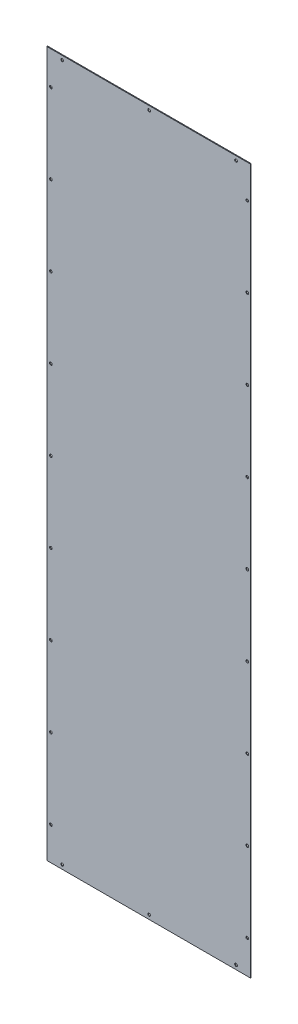
SolidWorks part; units mm, degrees
material "304"
ref_plane "前视基准面" through (0, 0, 0) normal (0, 0, 1) x (1, 0, 0)
ref_plane "上视基准面" through (0, 0, 0) normal (0, 1, 0) x (1, 0, 0)
ref_plane "右视基准面" through (0, 0, 0) normal (1, 0, 0) x (0, 0, -1)
sketch "草图1" plane through (0, 0, 0) normal (0, 0, 1) x (1, 0, 0)
  line L0 (0, 0) -> (451.2544, 0) construction
  line L1 (-247.25, 851.5) -> (247.25, 851.5)
  line L2 (-247.25, 851.5) -> (-247.25, -851.5)
  line L3 (-247.25, -851.5) -> (247.25, -851.5)
  line L4 (247.25, 851.5) -> (247.25, -851.5)
  line L5 (-247.25, 851.5) -> (247.25, -851.5) construction
  line L6 (-247.25, -851.5) -> (247.25, 851.5) construction
  line L7 (0, 0) -> (0, 412.8629) construction
  circle A0 centre (-237.25, 0) radius 3.25
  circle A1 centre (-237.25, -192.875) radius 3.25
  circle A2 centre (-237.25, -385.75) radius 3.25
  circle A3 centre (-237.25, -578.625) radius 3.25
  circle A4 centre (-237.25, -771.5) radius 3.25
  circle A34 centre (0, -841.5) radius 3.25
  circle A35 centre (0, 841.5) radius 3.25
  circle A36 centre (-237.25, 771.5) radius 3.25
  circle A37 centre (-237.25, 578.625) radius 3.25
  circle A38 centre (-237.25, 385.75) radius 3.25
  circle A39 centre (-237.25, 192.875) radius 3.25
  circle A40 centre (237.25, 192.875) radius 3.25
  circle A41 centre (237.25, 385.75) radius 3.25
  circle A42 centre (237.25, 578.625) radius 3.25
  circle A43 centre (237.25, 771.5) radius 3.25
  circle A44 centre (237.25, -771.5) radius 3.25
  circle A45 centre (237.25, -578.625) radius 3.25
  circle A46 centre (237.25, -385.75) radius 3.25
  circle A47 centre (237.25, -192.875) radius 3.25
  circle A48 centre (237.25, 0) radius 3.25
  circle A49 centre (-210, 841.5) radius 3.25
  circle A50 centre (210, 841.5) radius 3.25
  circle A51 centre (-210, -841.5) radius 3.25
  circle A52 centre (210, -841.5) radius 3.25
  point P0 (0, 0)
  point P49 (0, 0)
  point P50 (0, 0)
  dimension "D3" = 6.5
  dimension "D8" = 420
  dimension "D1" = 494.5
  dimension "D2" = 1703
  dimension "D4" = 10
  dimension "D6" = 10
  dimension "D7" = 80
  dimension "D5" = 5
extrude "凸台-拉伸1" add sketch "草图1" along normal blind 2
sketch "草图2" plane through (0, -851.5, 0) normal (0, -1, 0) x (-1, 0, 0)
  line L0 (247.25, 0) -> (-247.25, 0) construction
  line L1 (-247.25, -2) -> (-244.75, -2)
  line L2 (-247.25, -2) -> (-247.25, 0)
  line L3 (-247.25, 0) -> (-244.75, 0)
  line L4 (-244.75, -2) -> (-244.75, 0)
  dimension "D1" = 2.5
extrude "切除-拉伸1" cut sketch "草图2" against normal through all
